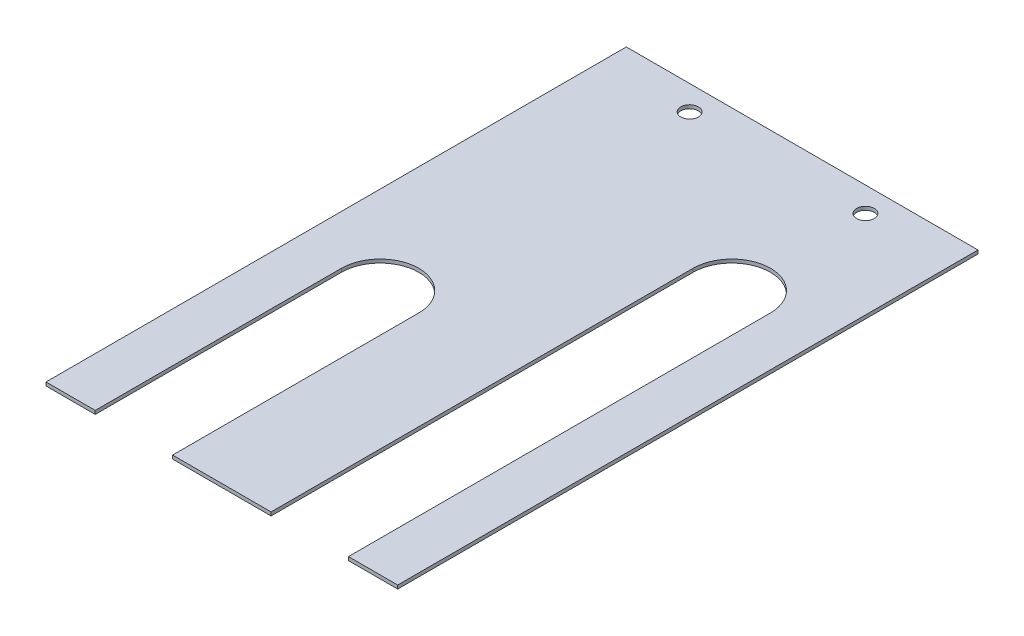
from build123d import *

# Parameters (mm, degrees)
SKETCH_1_W          = 100
SKETCH_1_H          = 165
EXTRUDE_1_DEPTH     = 1
SKETCH_2_R          = 2.5
CUT_EXTRUDE_1_DEPTH = 97.474089786


with BuildPart() as part:
    # 草图1 → 凸台-拉伸1 (new body)
    with BuildSketch(Plane(origin=(0, 0, 0), x_dir=(1, 0, 0), z_dir=(0, 1, 0))):
        Rectangle(SKETCH_1_W, SKETCH_1_H)
    extrude(amount=EXTRUDE_1_DEPTH)

    # 草图2 → 切除-拉伸1 (cut, through all)
    with BuildSketch(Plane(origin=(0, 1, 0), x_dir=(1, 0, 0), z_dir=(0, 1, 0))):
        with Locations(Location((-25, 75.5, 0), (0, 0, 270))):
            Circle(SKETCH_2_R)
        with Locations(Location((25, 75.5, 0), (0, 0, 270))):
            Circle(SKETCH_2_R)
        with BuildLine():
            Line((-36, -82.5), (-36, -12.5))
            ThreePointArc((-36, -12.5), (-25, -1.5), (-14, -12.5))
            Line((-14, -12.5), (-14, -82.5))
            ThreePointArc((-14, -82.5), (-25, -93.5), (-36, -82.5))
        make_face()
        with BuildLine():
            Line((14, -82.5), (14, 37.5))
            ThreePointArc((14, 37.5), (25, 48.5), (36, 37.5))
            Line((36, 37.5), (36, -82.5))
            ThreePointArc((36, -82.5), (25, -93.5), (14, -82.5))
        make_face()
    extrude(amount=-CUT_EXTRUDE_1_DEPTH, mode=Mode.SUBTRACT)


solid = part.part
